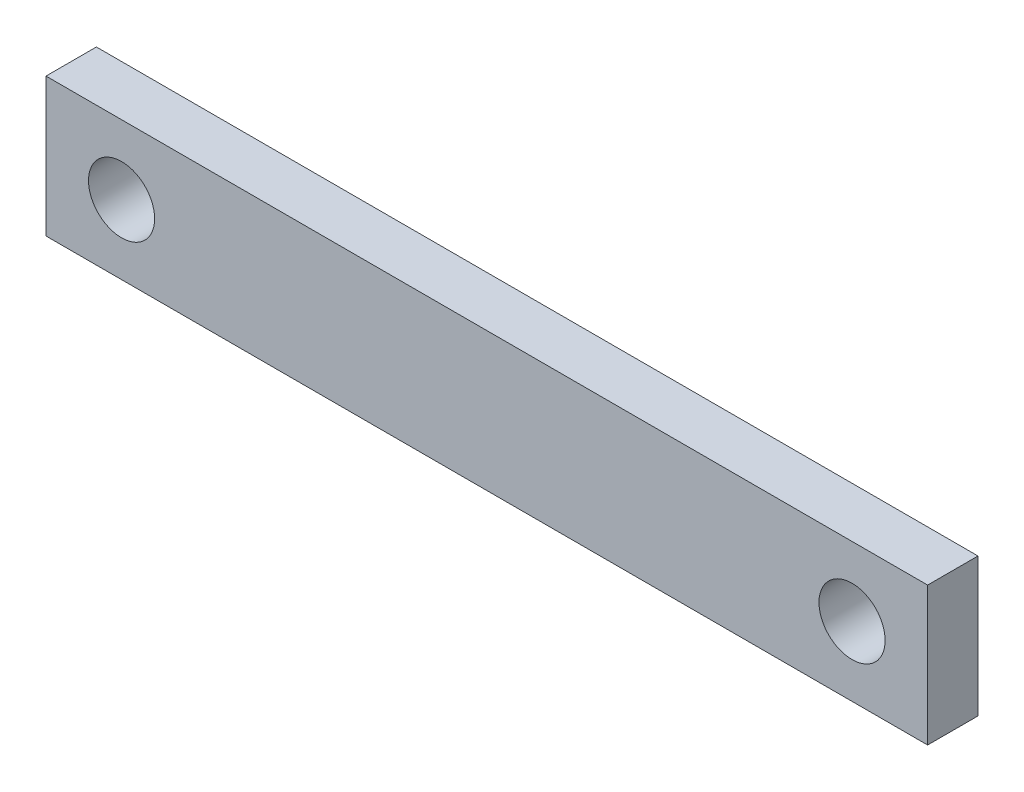
from build123d import *

# Parameters (mm, degrees)
SKETCH1_W           = 140
SKETCH1_H           = 22
BOSS_EXTRUDE1_DEPTH = 8
SKETCH2_R           = 5.25
CUT_EXTRUDE1_DEPTH  = 79.751224998


with BuildPart() as part:
    # Sketch1 → Boss-Extrude1 (new body)
    with BuildSketch(Plane.XY):
        with Locations((0.089565278, 24.00297527)):
            Rectangle(SKETCH1_W, SKETCH1_H)
    extrude(amount=BOSS_EXTRUDE1_DEPTH)

    # Sketch2 → Cut-Extrude1 (cut, through all)
    with BuildSketch(Plane.XY.offset(8)):
        with Locations((-57.910434722, 24.00297527)):
            Circle(SKETCH2_R)
        with Locations(Location((58.089565278, 24.00297527, 0), (0, 0, 180))):
            Circle(SKETCH2_R)
    extrude(amount=-CUT_EXTRUDE1_DEPTH, mode=Mode.SUBTRACT)


solid = part.part
